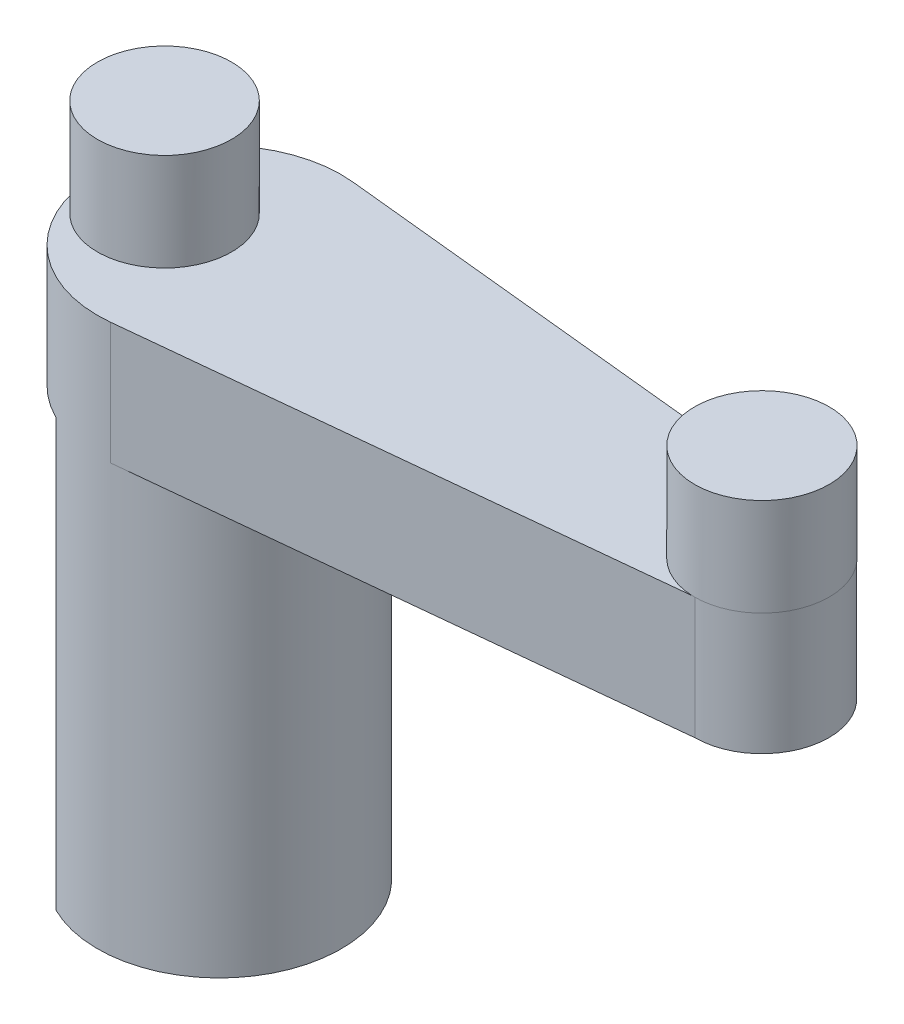
from build123d import *

# Parameters (mm, degrees)
EXTRUDE_1_DEPTH = 1
SKETCH_2_R      = 0.552067548
SKETCH_2_R_2    = 0.55
EXTRUDE_2_DEPTH = 0.8
EXTRUDE_START   = 3.5
EXTRUDE_3_DEPTH = 3.5
SCALE_1_SCALE   = 0.7


with BuildPart() as part:
    # 草图1 → 凸台-拉伸1 (new body)
    with BuildSketch(Plane(origin=(0, 0, 0), x_dir=(1, 0, 0), z_dir=(0, 1, 0))):
        with BuildLine():
            Line((0.101765249, -0.994808441), (4.45, -0.55))
            ThreePointArc((4.45, -0.55), (5, 0), (4.45, 0.55))
            Line((4.45, 0.55), (0.101765249, 0.994808441))
            ThreePointArc((0.101765249, 0.994808441), (-1, 0), (0.101765249, -0.994808441))
        make_face()
    extrude(amount=EXTRUDE_1_DEPTH)

    # 草图2 → 凸台-拉伸2 (add)
    with BuildSketch(Plane(origin=(0, 1, 0), x_dir=(1, 0, 0), z_dir=(0, 1, 0))):
        with Locations(Location((4.45, 0, 0), (0, 0, 91.816467299))):
            Circle(SKETCH_2_R)
        with Locations(Location((-0.45, 0, 0), (0, 0, 179.998371267))):
            Circle(SKETCH_2_R_2)
    extrude(amount=EXTRUDE_2_DEPTH)

    # 草图3 → 凸台-拉伸3 (add)
    with BuildSketch(Plane.XZ.offset(EXTRUDE_START)):
        with BuildLine():
            Line((0.258819045, -0.965925826), (-0.181173332, 0.676148078))
            Line((-0.181173332, 0.676148078), (-0.374358497, 0.624384269))
            Line((-0.374358497, 0.624384269), (-0.446775004, 0.894646352))
            ThreePointArc((-0.446775004, 0.894646352), (0.935020892, 0.354592627), (0.258819045, -0.965925826))
        make_face()
    extrude(amount=-EXTRUDE_3_DEPTH)


with BuildPart() as part_1:
    # 缩放比例1: scaled about (1.278779504, -0.207492691, 0.047331659)
    add(part.part.scale(SCALE_1_SCALE).moved(Location((0.383633851, -0.062247807, 0.014199498))))


solid = part_1.part
